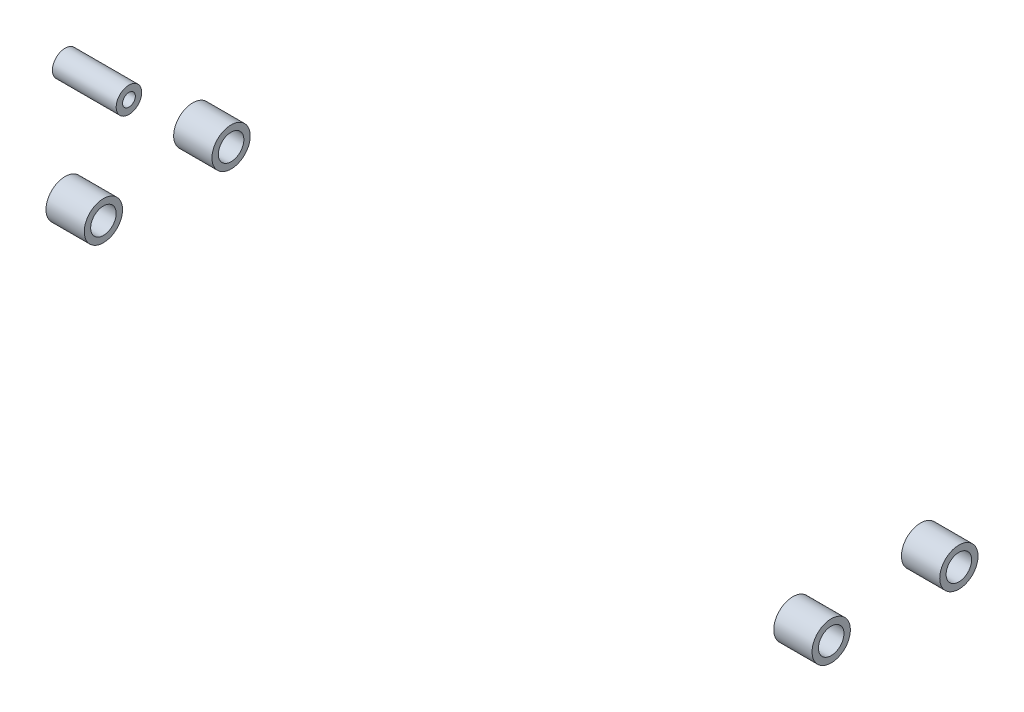
SolidWorks part; units mm, degrees
material "普通碳钢"
ref_plane "Front Plane" through (0, 0, 0) normal (0, 0, 1) x (1, 0, 0)
ref_plane "Top Plane" through (0, 0, 0) normal (0, 1, 0) x (1, 0, 0)
ref_plane "Right Plane" through (0, 0, 0) normal (1, 0, 0) x (0, 0, -1)
sketch "Sketch1" plane through (0, 0, 0) normal (0, 0, 1) x (1, 0, 0)
  line L0 (-367.3808, 0) -> (382.5816, 0) construction
  line L1 (-300, 15) -> (-300, 10)
  line L2 (-300, 10) -> (-270, 10)
  line L3 (-270, 10) -> (-270, 15)
  line L4 (-270, 15) -> (-300, 15)
  line L5 (270, 15) -> (270, 10)
  line L6 (270, 10) -> (300, 10)
  line L7 (300, 10) -> (300, 15)
  line L8 (300, 15) -> (270, 15)
  dimension "D1" = 300
  dimension "D2" = 600
  dimension "D3" = 10
  dimension "D4" = 5
  dimension "D5" = 30
  dimension "D6" = 30
  dimension "D7" = 5
  dimension "D8" = 10
revolve "Revolve1" add sketch "Sketch1" angle 360 about L0
ref_plane "Plane1" through (0, 0, 50) normal (0, 0, 1) x (1, 0, 0)
mirror "Mirror5" about plane through (0, 0, 50) normal (0, 0, 1) of bodies 106 107
sketch "Sketch3" plane through (-300, 0, 0) normal (-1, 0, 0) x (0, 0, 1)
  circle A0 centre (50, 42) radius 10
  circle A1 centre (50, 42) radius 5
  circle A2 centre (0, 0) radius 10 construction
  dimension "D1" = 50
  dimension "D2" = 42
  dimension "D3" = 20
  dimension "D4" = 10
extrude "Boss-Extrude1" add sketch "Sketch3" along normal blind 50 separate body
